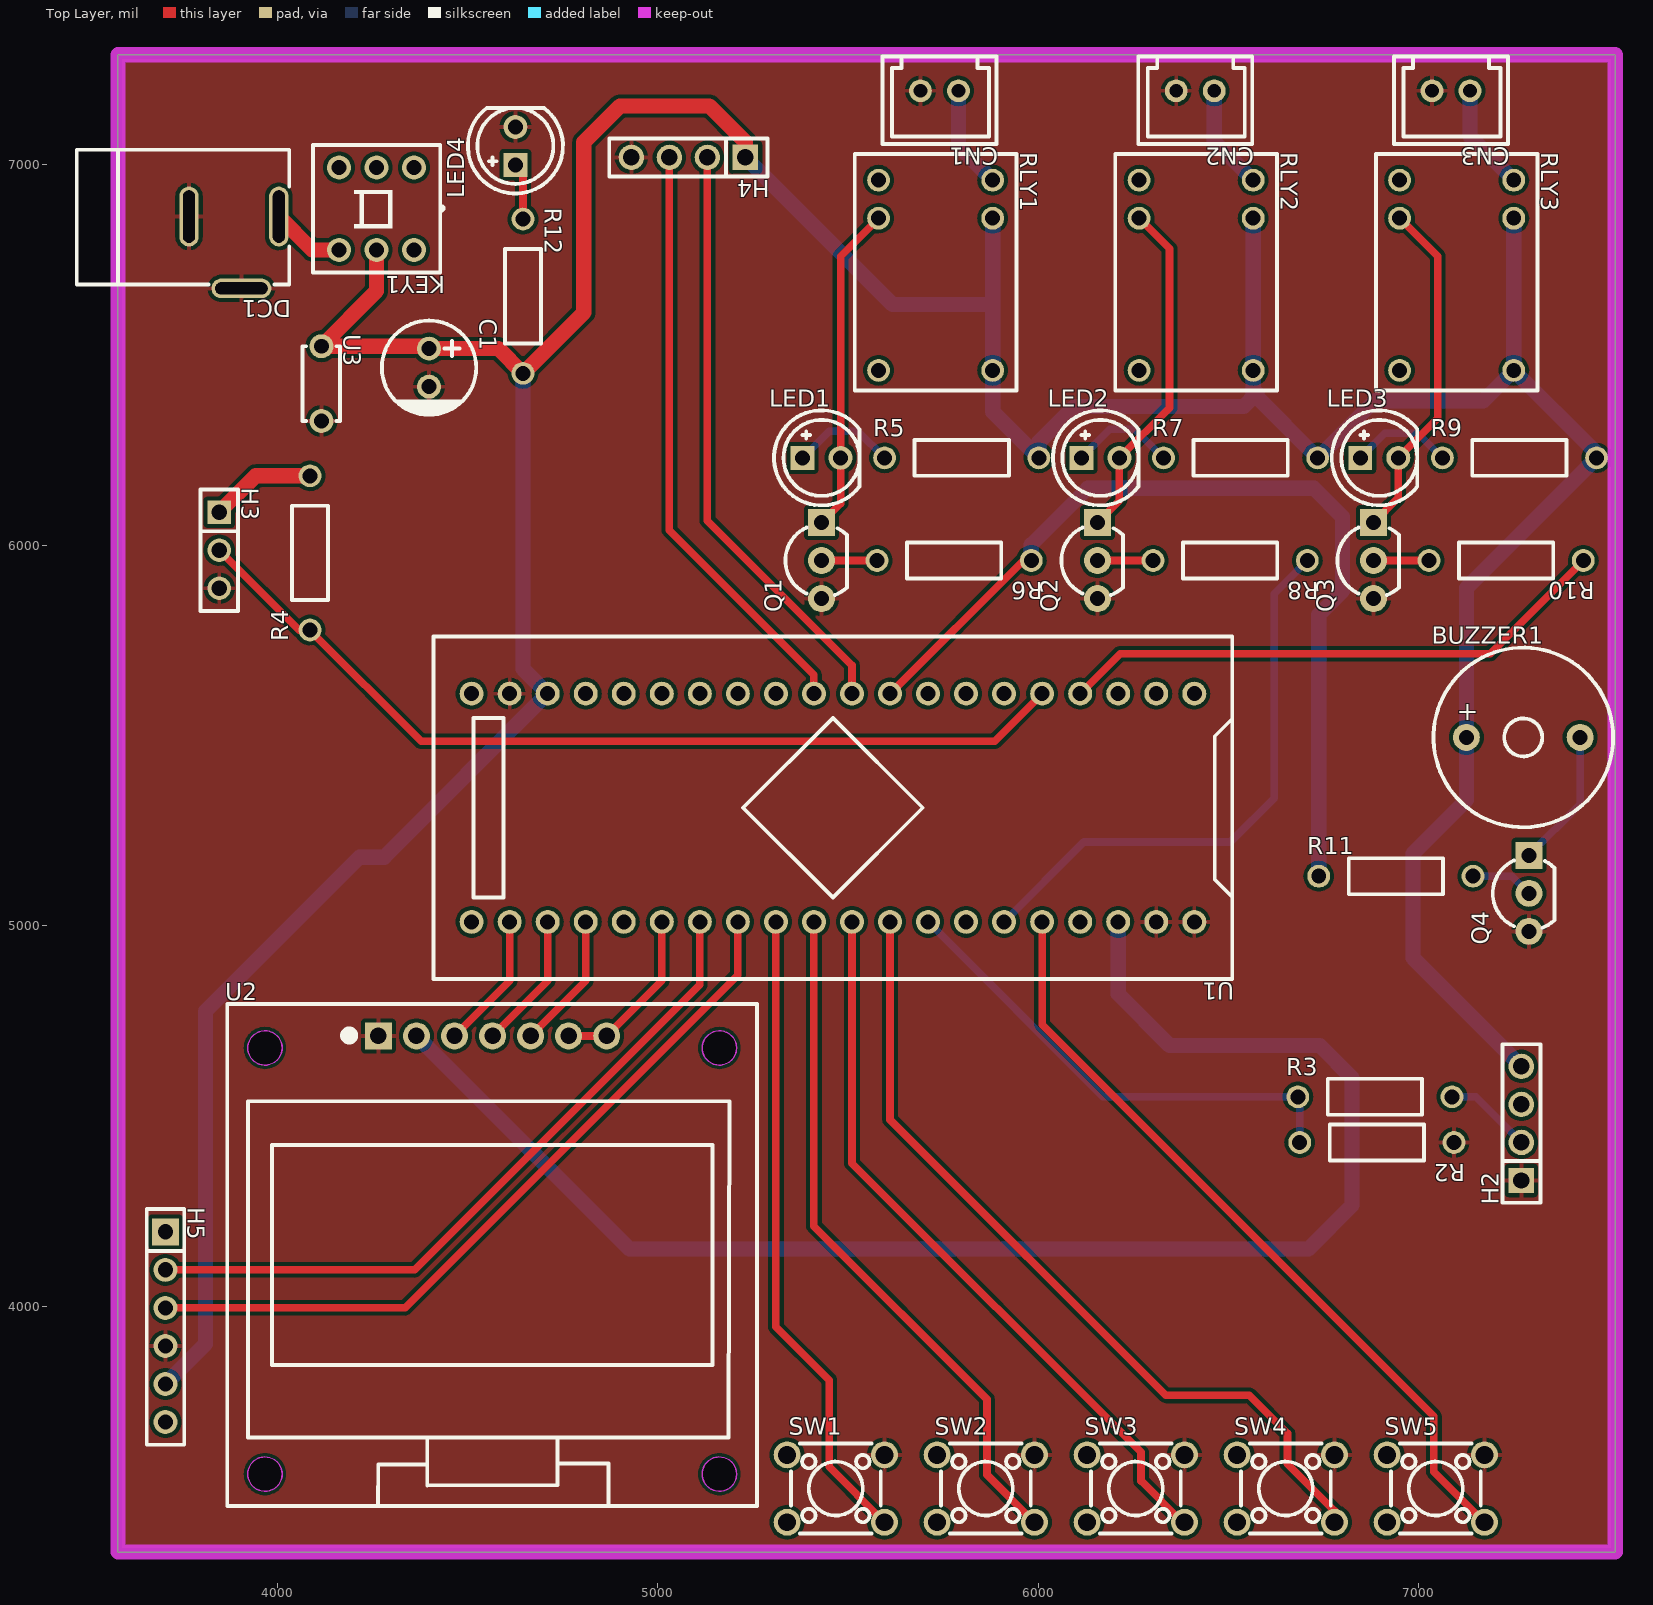
[diagram p0: Top Layer view]
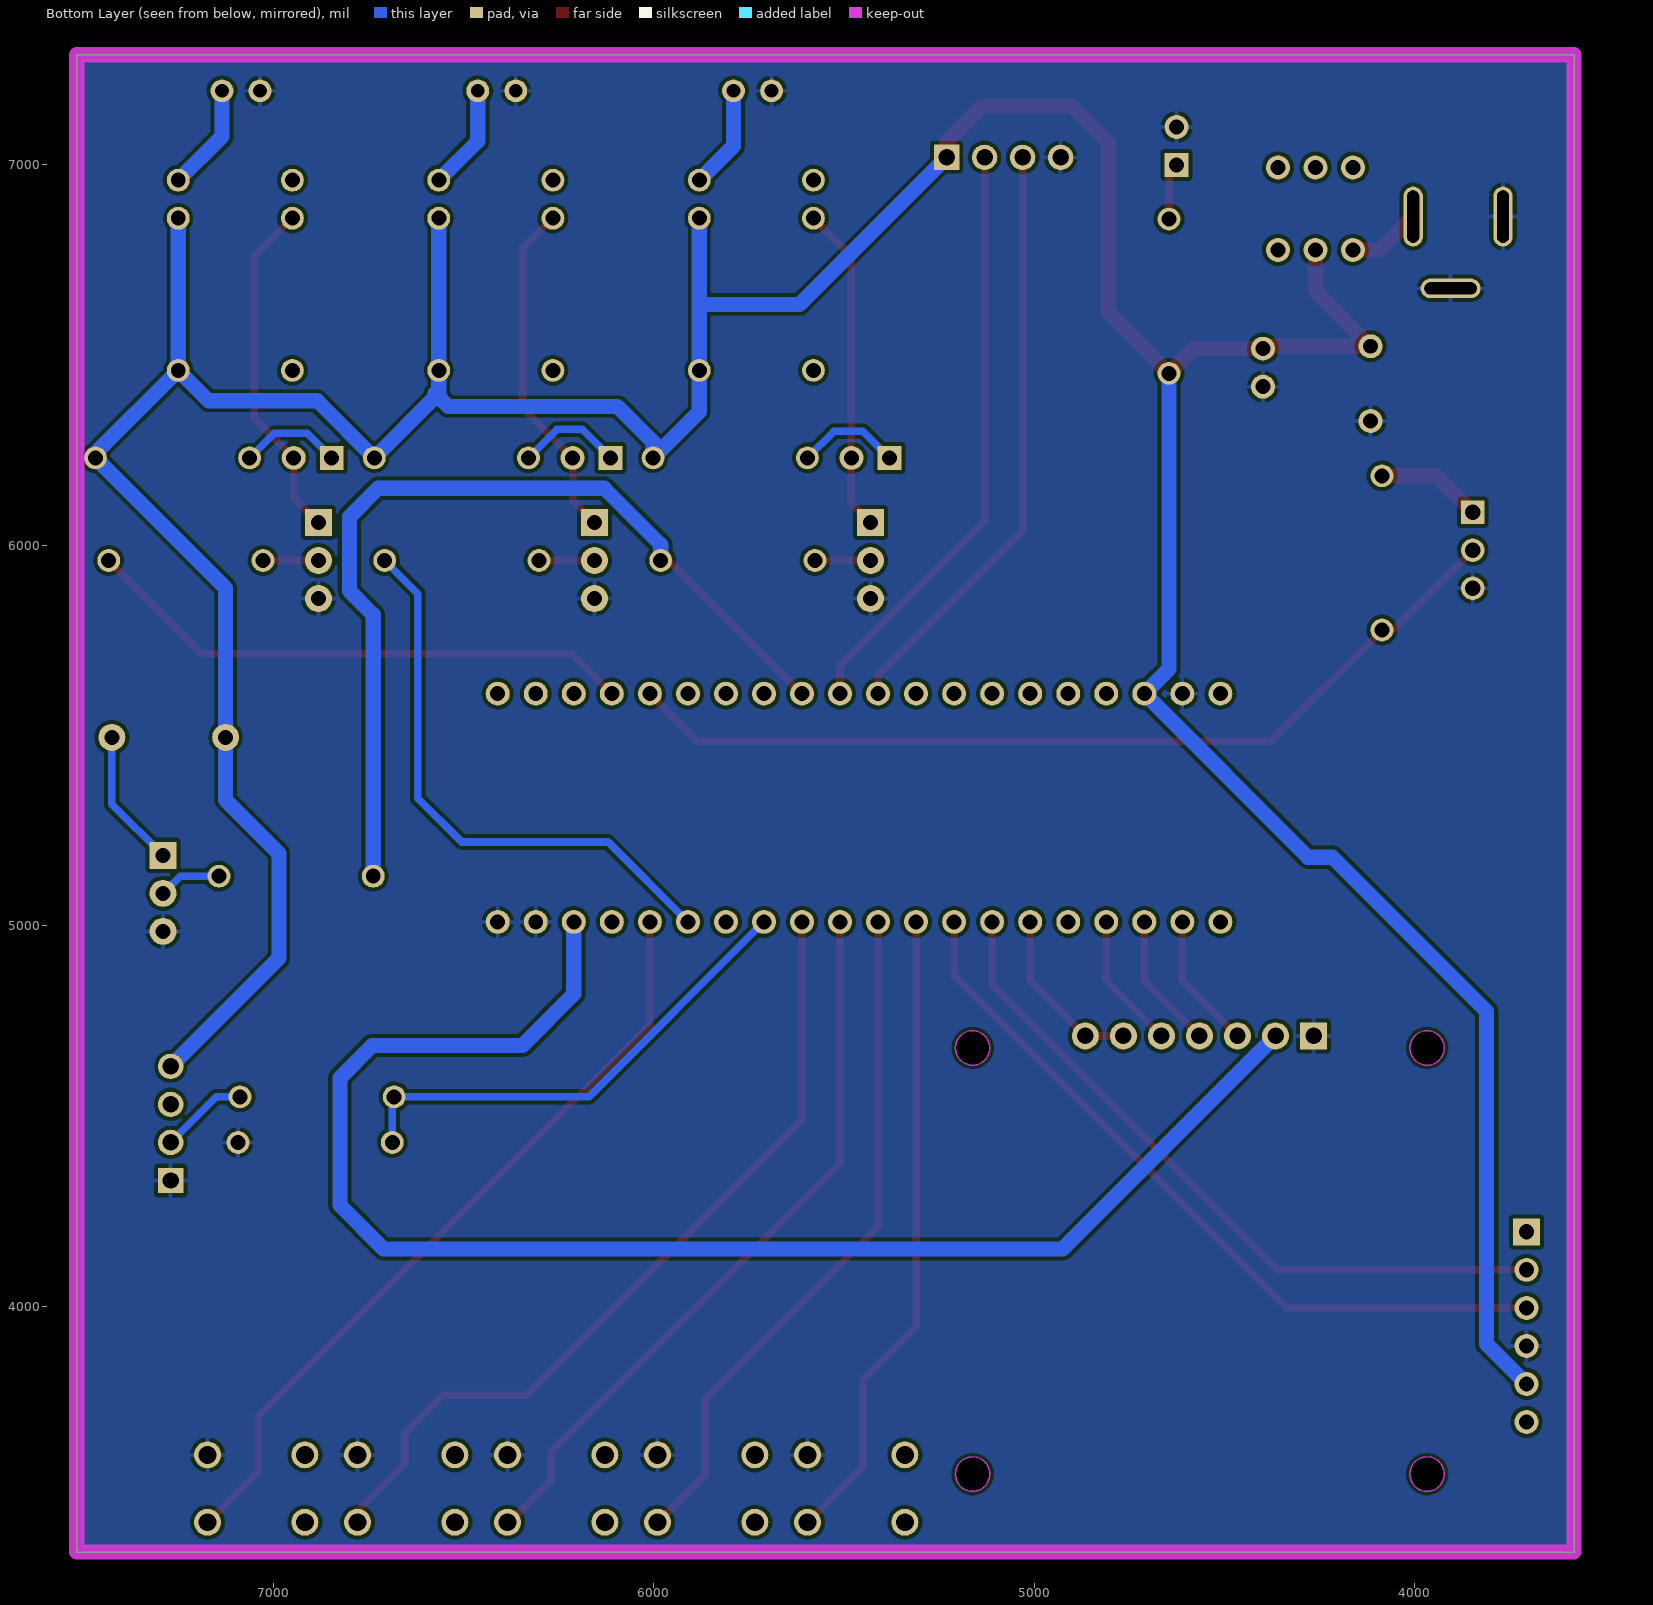
[diagram p1: Bottom Layer view, seen from below]
# Altium PCB MISC50991.pcbdoc
Units mil, origin at the board's own origin, x right, y up, seen from the top; angles counter-clockwise.
Board outline 3937.01 x 3937.01 mil, 2 copper layers (Top Layer, Bottom Layer), stack 62.206 mil thick; 41 components, 56 nets, 165 pads, 0 vias.

## Layer stack, top to bottom
Top Solder Mask Layer: solder mask 0.394, Dk 3.3
Top Layer: signal copper 1.379
Dielectric1: surface 59.449, FR4, Dk 4.5
Bottom Layer: signal copper 1.378
Bottom Solder Mask Layer: solder mask 0.394, Dk 3.3

## Board outline
3580,7290 3580,3352.99 7517.01,3352.99 7517.01,7290

## Design rules (kind name [scope] priority, off if disabled: settings)
BoardOutlineClearance copperThickness2oz_1 [All] p2 off: genericclearance=7.99 ignorepadtopadclearanceinfootprint=FALSE except(0: Arc-SplitContinuation Track-SplitContinuation SMDPad-SplitContinuation THPad-SplitContinuation Via-SplitContinuation Fill-SplitContinuation Region-SplitContinuation Poly-SplitContinuation Text-SplitContinuation Hole-SplitContinuation; 5.98: Arc-CutoutEdge Track-CutoutEdge SMDPad-CutoutEdge THPad-CutoutEdge Via-CutoutEdge Text-CutoutEdge; 6.9: Hole-OutlineEdge Hole-CutoutEdge; 10: Poly-OutlineEdge Poly-CutoutEdge; 11.81: Arc-OutlineEdge Track-OutlineEdge SMDPad-OutlineEdge THPad-OutlineEdge Via-OutlineEdge Fill-OutlineEdge Region-OutlineEdge Text-OutlineEdge Fill-CutoutEdge Region-CutoutEdge)
BoardOutlineClearance Plane_innerPlane_1 [All] p4 off: genericclearance=4.02 ignorepadtopadclearanceinfootprint=FALSE except(0: Arc-SplitContinuation Track-SplitContinuation SMDPad-SplitContinuation THPad-SplitContinuation Via-SplitContinuation Fill-SplitContinuation Region-SplitContinuation Poly-SplitContinuation Text-SplitContinuation Hole-SplitContinuation; 5.98: Arc-CutoutEdge Track-CutoutEdge SMDPad-CutoutEdge THPad-CutoutEdge Via-CutoutEdge Text-CutoutEdge; 6.9: Hole-OutlineEdge Hole-CutoutEdge; 10: Poly-OutlineEdge Poly-CutoutEdge; 11.81: Arc-OutlineEdge Track-OutlineEdge SMDPad-OutlineEdge THPad-OutlineEdge Via-OutlineEdge Fill-OutlineEdge Region-OutlineEdge Text-OutlineEdge Fill-CutoutEdge Region-CutoutEdge)
BoardOutlineClearance Copper_copperRegion_1 [All] p6 off: genericclearance=4.02 ignorepadtopadclearanceinfootprint=FALSE except(0: Arc-SplitContinuation Track-SplitContinuation SMDPad-SplitContinuation THPad-SplitContinuation Via-SplitContinuation Fill-SplitContinuation Region-SplitContinuation Poly-SplitContinuation Text-SplitContinuation Hole-SplitContinuation; 5.98: Arc-CutoutEdge Track-CutoutEdge SMDPad-CutoutEdge THPad-CutoutEdge Via-CutoutEdge Text-CutoutEdge; 6.9: Hole-OutlineEdge Hole-CutoutEdge; 10: Poly-OutlineEdge Poly-CutoutEdge; 11.81: Arc-OutlineEdge Track-OutlineEdge SMDPad-OutlineEdge THPad-OutlineEdge Via-OutlineEdge Fill-OutlineEdge Region-OutlineEdge Text-OutlineEdge Fill-CutoutEdge Region-CutoutEdge)
BoardOutlineClearance copperThickness1oz_1 [All] p8: genericclearance=4.02 ignorepadtopadclearanceinfootprint=FALSE except(0: Arc-SplitContinuation Track-SplitContinuation SMDPad-SplitContinuation THPad-SplitContinuation Via-SplitContinuation Fill-SplitContinuation Region-SplitContinuation Poly-SplitContinuation Text-SplitContinuation Hole-SplitContinuation; 5.98: Arc-CutoutEdge Track-CutoutEdge SMDPad-CutoutEdge THPad-CutoutEdge Via-CutoutEdge Text-CutoutEdge; 6.9: Hole-OutlineEdge Hole-CutoutEdge; 10: Poly-OutlineEdge Poly-CutoutEdge; 11.81: Arc-OutlineEdge Track-OutlineEdge SMDPad-OutlineEdge THPad-OutlineEdge Via-OutlineEdge Fill-OutlineEdge Region-OutlineEdge Text-OutlineEdge Fill-CutoutEdge Region-CutoutEdge)
Clearance copperThickness2oz [All] p1 off: gap=7.99 ignorepadtopadclearanceinfootprint=FALSE except(5.98: SMDPad-Track SMDPad-SMDPad THPad-Track SMDPad-THPad THPad-THPad Track-Via SMDPad-Via THPad-Via Via-Via Fill-SMDPad Region-SMDPad Fill-THPad Region-THPad Fill-Via Region-Via Fill-Fill Fill-Region Region-Region Arc-Track Arc-SMDPad Arc-THPad Arc-Via Fill-Arc Region-Arc Arc-Arc Text-Track SMDPad-Text Text-THPad Text-Via Fill-Text Region-Text Arc-Text Text-Text; 6.9: Hole-Track Hole-SMDPad Hole-THPad Hole-Via Fill-Hole Region-Hole Hole-Arc Hole-Text; 10: Poly-Track Poly-SMDPad Poly-THPad Poly-Via Poly-Fill Poly-Region Poly-Poly Poly-Arc Poly-Text Poly-Hole; 11.81: Fill-Track Region-Track)
Clearance Plane_innerPlane [All] p3 off: gap=4.02 ignorepadtopadclearanceinfootprint=FALSE except(5.98: SMDPad-Track SMDPad-SMDPad THPad-Track SMDPad-THPad THPad-THPad Track-Via SMDPad-Via THPad-Via Via-Via Fill-SMDPad Region-SMDPad Fill-THPad Region-THPad Fill-Via Region-Via Fill-Fill Fill-Region Region-Region Arc-Track Arc-SMDPad Arc-THPad Arc-Via Fill-Arc Region-Arc Arc-Arc Text-Track SMDPad-Text Text-THPad Text-Via Fill-Text Region-Text Arc-Text Text-Text; 6.9: Hole-Track Hole-SMDPad Hole-THPad Hole-Via Fill-Hole Region-Hole Hole-Arc Hole-Text; 10: Poly-Track Poly-SMDPad Poly-THPad Poly-Via Poly-Fill Poly-Region Poly-Poly Poly-Arc Poly-Text Poly-Hole; 11.81: Fill-Track Region-Track)
Clearance Copper_copperRegion [All] p5 off: gap=4.02 ignorepadtopadclearanceinfootprint=FALSE except(5.98: SMDPad-Track SMDPad-SMDPad THPad-Track SMDPad-THPad THPad-THPad Track-Via SMDPad-Via THPad-Via Via-Via Fill-SMDPad Region-SMDPad Fill-THPad Region-THPad Fill-Via Region-Via Fill-Fill Fill-Region Region-Region Arc-Track Arc-SMDPad Arc-THPad Arc-Via Fill-Arc Region-Arc Arc-Arc Text-Track SMDPad-Text Text-THPad Text-Via Fill-Text Region-Text Arc-Text Text-Text; 6.9: Hole-Track Hole-SMDPad Hole-THPad Hole-Via Fill-Hole Region-Hole Hole-Arc Hole-Text; 10: Poly-Track Poly-SMDPad Poly-THPad Poly-Via Poly-Fill Poly-Region Poly-Poly Poly-Arc Poly-Text Poly-Hole; 11.81: Fill-Track Region-Track)
Clearance copperThickness1oz [All] p7: gap=4.02 ignorepadtopadclearanceinfootprint=FALSE except(5.98: SMDPad-Track SMDPad-SMDPad THPad-Track SMDPad-THPad THPad-THPad Track-Via SMDPad-Via THPad-Via Via-Via Fill-SMDPad Region-SMDPad Fill-THPad Region-THPad Fill-Via Region-Via Fill-Fill Fill-Region Region-Region Arc-Track Arc-SMDPad Arc-THPad Arc-Via Fill-Arc Region-Arc Arc-Arc Text-Track SMDPad-Text Text-THPad Text-Via Fill-Text Region-Text Arc-Text Text-Text; 6.9: Hole-Track Hole-SMDPad Hole-THPad Hole-Via Fill-Hole Region-Hole Hole-Arc Hole-Text; 10: Poly-Track Poly-SMDPad Poly-THPad Poly-Via Poly-Fill Poly-Region Poly-Poly Poly-Arc Poly-Text Poly-Hole; 11.81: Fill-Track Region-Track)
DiffPairsRouting differentialPair [All] p1: maxlimit=6 minlimit=6 mostfreqgap=6 toplayer_minwidth=5 toplayer_prefwidth=10 toplayer_maxwidth=100 toplayer_mingap=6 toplayer_prefgap=6 toplayer_maxgap=6 bottomlayer_minwidth=5 bottomlayer_prefwidth=10 bottomlayer_maxwidth=100 bottomlayer_mingap=6 bottomlayer_prefgap=6 bottomlayer_maxgap=6 maxuncoupledlength=10
HoleToHoleClearance otherClearance [All] p1: gap=11.81 allowstackedmicrovias=TRUE
Length netLength [All] p1: minlimit=0 maxlimit=0
PasteMaskExpansion pasteMaskExpansion [All] p1: expansion=0
PlaneConnect innerPlane [All] p1: planeconnectstyle=Relief reliefexpansion=20 reliefentries=4 reliefconductorwidth=10 reliefairgap=10
PolygonConnect copperRegion [All] p1: connectstyle=Relief reliefconductorwidth=10 reliefentries=4 polygonreliefangle="90 Angle" airgapwidth=10 via.connectstyle=Relief via.reliefconductorwidth=10 via.reliefentries=4 via.polygonreliefangle="90 Angle" via.airgapwidth=10
RoutingVias viaSize [All] p1: holewidth=12.01 width=24.02 viastyle="Through Hole" minholewidth=11.81 minwidth=19.68 maxholewidth=248.03 maxwidth=393.7
SolderMaskExpansion solderMaskExpansion [IsVia] p1: expansion=-1000 istentingtop=TRUE
SolderMaskExpansion solderMaskExpansion [All] p2: expansion=2 istentingtop=FALSE
Width copperThickness2oz_2 [All] p1 off: maxlimit=100 minlimit=8 preferedwidth=10
Width copperThickness1oz_2 [All] p2: maxlimit=100 minlimit=5 preferedwidth=10

## Components (designator, comment, footprint, x,y, rotation, side; value= is the part's Value field where it differs from the comment)
BUZZER1 "buzzer-12X9" BUZ-TH_BD12.0-P7.60-D0.6-FD 7275,5495 r0 top
C1 "220uF" CAP-TH_BD6.3-P2.50-D1.0-FD 4398,6467.12 r270 top
CN1 "2P PH2.54" CONN-TH_2P-P2.54_HDR2 5740,7195 r180 top
CN2 "2P PH2.54" CONN-TH_2P-P2.54_HDR2 6412.5,7195 r180 top
CN3 "2P PH2.54" CONN-TH_2P-P2.54_HDR2 7085,7195 r180 top
DC1 "" DC-2.0 3880,6875 r180 top
H2 "" HDR-TH_4P-P2.54-V-F 7270,4480 r90 top
H3 "" HDR-TH_3P-P2.54-V-F 3846.54,5987.12 r270 top
H4 "" HDR-TH_4P-P2.54-V-F 5080,7020 r180 top
H5 "" HDR-TH_6P-P2.54-V-F 3705,3945 r270 top
KEY1 "Non-latching switch 8.5×8.5 silent" SW-TH_6P-L8.5-W8.5-P2.54 4260,6885 r180 top
LED1 "" LED-TH_5mm 5430,6230 r0 top
LED2 "" LED-TH_5mm 6163.21,6230 r0 top
LED3 "" LED-TH_5mm 6896.43,6230 r0 top
LED4 "" LED-TH_5mm 4625,7050 r90 top
Q1 "9013" TO-92-3_L4.8-W3.7-P2.54-R 5430,5960 r90 top
Q2 "9013" TO-92-3_L4.8-W3.7-P2.54-R 6155.64,5960 r90 top
Q3 "9013" TO-92-3_L4.8-W3.7-P2.54-R 6881.29,5960 r90 top
Q4 "9013" TO-92-3_L4.8-W3.7-P2.54-R 7290,5085 r90 top
R2 "10kΩ" Res_1/4W 6890,4430 r180 top
R3 "5kΩ" Res_1/4W 6885,4550 r0 top
R4 "5kΩ" Res_1/4W 4085,5980 r90 top
R5 "5kΩ" Res_1/4W 5798.57,6230 r0 top
R6 "5kΩ" Res_1/4W 5778.71,5960 r180 top
R7 "5kΩ" Res_1/4W 6531.79,6230 r0 top
R8 "5kΩ" Res_1/4W 6504.36,5960 r180 top
R9 "5kΩ" Res_1/4W 7265,6230 r0 top
R10 "5kΩ" Res_1/4W 7230,5960 r180 top
R11 "5kΩ" Res_1/4W 6940,5130 r0 top
R12 "5kΩ" Res_1/4W 4645,6655 r270 top
RLY1 "SRS-05VDC-SL-C" RELAY-TH_SRS-05VDC-SL-C 5730,6710 r270 top
RLY2 "SRS-05VDC-SL-C" RELAY-TH_SRS-05VDC-SL-C 6415,6710 r270 top
RLY3 "SRS-05VDC-SL-C" RELAY-TH_SRS-05VDC-SL-C 7100,6710 r270 top
SW1 "" SW-TH_4P-L6.0-W6.0-P4.50-LS6.5 5467.49,3520 r180 top
SW2 "" SW-TH_4P-L6.0-W6.0-P4.50-LS6.5 5861.87,3520 r180 top
SW3 "" SW-TH_4P-L6.0-W6.0-P4.50-LS6.5 6256.25,3520 r180 top
SW4 "" SW-TH_4P-L6.0-W6.0-P4.50-LS6.5 6650.62,3520 r180 top
SW5 "" SW-TH_4P-L6.0-W6.0-P4.50-LS6.5 7045,3520 r180 top
U1 "STM32F103C8T6-Card" CONN-TH_L53.3-W22.9_STM32F103C8T6-CARD 5460,5310 r180 top
U2 "1.30OLED_7P" LCD-TH_7P-P2.54_1.30OLED_7P 4565,4710 r0 top
U3 "100nF" CAP-TH_L5.0-W2.5-P5.00-D1.0 4115,6425 r270 top

## Footprints (in the part's own frame and the unit in brackets; to place one, negate y for a bottom-side part, rotate by r counter-clockwise, add the part's x,y. Pads: shape width x height; smd on the part's side, far side on the other; paste and mask are expansions set on the pad)
BUZ-TH_BD12.0-P7.60-D0.6-FD [mm]
  round 1.8 hole 1: 1(-3.8,0) 2(3.8,0)
  silkscreen extent -6,-6 6,6
CAP-TH_BD6.3-P2.50-D1.0-FD [mm]
  round 1.6 hole 1: 1(-1.27,0) 2(1.27,0)
  silkscreen extent -3.15,-3.15 3.17,3.15
CAP-TH_L5.0-W2.5-P5.00-D1.0 [mm]
  round 1.6 hole 1: 1(-2.5,0) 2(2.5,0)
  silkscreen extent -2.5,-1.27 2.5,1.25
CONN-TH_2P-P2.54_HDR2 [mil]
  round 60 hole 36 paste+0 mask+1.97: 1(-50,0) 2(50,0)
  silkscreen extent -150,-90 150,140
CONN-TH_L53.3-W22.9_STM32F103C8T6-CARD [mm]
  round 1.6 hole 1: 1(-24.13,-7.62) 2(-21.59,-7.62) 3(-19.05,-7.62) 4(-16.51,-7.62) 5(-13.97,-7.62) 6(-11.43,-7.62) 7(-8.89,-7.62) 8(-6.35,-7.62) 9(-3.81,-7.62) 10(-1.27,-7.62) 11(1.27,-7.62) 12(3.81,-7.62) 13(6.35,-7.62) 14(8.89,-7.62) 15(11.43,-7.62) 16(13.97,-7.62) 17(16.51,-7.62) 18(19.05,-7.62) 19(21.59,-7.62) 20(24.13,-7.62) 21(24.13,7.62) 22(21.59,7.62) 23(19.05,7.62) 24(16.51,7.62) 25(13.97,7.62) 26(11.43,7.62) 27(8.89,7.62) 28(6.35,7.62) 29(3.81,7.62) 30(1.27,7.62) 31(-1.27,7.62) 32(-3.81,7.62) 33(-6.35,7.62) 34(-8.89,7.62) 35(-11.43,7.62) 36(-13.97,7.62) 37(-16.51,7.62) 38(-19.05,7.62) 39(-21.59,7.62) 40(-24.13,7.62)
  silkscreen extent -26.67,-11.43 26.67,11.43
DC-2.0 [mil]
  oval 157.5x51.2 hole 31.5 slot 137.8 at 0 deg paste+0 mask+2: 2(-24.7,199.5)
  oval 51.2x157.5 hole 31.5 slot 137.8 at 90 deg paste+0 mask+2: 3(113.1,10.5) 4(-123.1,10.5)
  silkscreen extent -151,-165 408,190
HDR-TH_3P-P2.54-V-F [mil]
  rect 62x62 hole 40.16: 1(-100,0)
  round 62 hole 40.16: 2(0,0) 3(100,0)
  silkscreen extent -160,-49 160,49
HDR-TH_4P-P2.54-V-F [mm]
  rect 1.7x1.7 hole 1.1: 1(-3.81,0)
  round 1.7 hole 1.1: 2(-1.27,0) 3(1.27,0) 4(3.81,0)
  silkscreen extent -5.29,-1.27 5.29,1.27
HDR-TH_6P-P2.54-V-F [mm]
  rect 1.8x1.8 hole 1.02: 1(-6.35,0)
  round 1.6 hole 1.02: 2(-3.81,0) 3(-1.27,0) 4(1.27,0) 5(3.81,0) 6(6.35,0)
  silkscreen extent -7.87,-1.25 7.87,1.25
LCD-TH_7P-P2.54_1.30OLED_7P [mil]
  rect 70.94x70.94 hole 43.3: 1(-300,-0.01)
  round 70.94 hole 43.3: 2(-200,-0.01) 3(-100,-0.01) 4(0,-0.01) 5(100,-0.01) 6(200,-0.01) 7(300,-0.01)
  Board Outline Layer circle w0.1: c-598.44,-31.49 r45.28
  Board Outline Layer circle w0.1: c596.44,-1151.96 r45.28
  Board Outline Layer circle w0.1: c596.44,-31.49 r45.28
  Board Outline Layer circle w0.1: c-598.44,-1151.96 r45.28
  Board Outline Layer region: -553.17,-31.49 -557.65,-51.14 -570.21,-66.89 -588.37,-75.63 -608.52,-75.63 -626.67,-66.89 -639.23,-51.14 -643.72,-31.49 -643.72,-31.49 -639.23,-11.85 -626.67,3.91 -608.52,12.65 -588.37,12.65 -570.21,3.91 -557.65,-11.85 -553.17,-31.49
  Board Outline Layer region: -553.17,-31.49 -553.55,-37.4 -554.71,-43.21 -556.61,-48.82 -559.23,-54.13 -562.52,-59.06 -566.43,-63.51 -570.88,-67.41 -575.8,-70.7 -581.12,-73.32 -586.72,-75.23 -592.53,-76.38 -598.44,-76.77 -604.35,-76.38 -610.16,-75.23 -615.77,-73.32 -621.08,-70.7 -626,-67.41 -630.46,-63.51 -634.36,-59.06 -637.65,-54.13 -640.27,-48.82 -642.18,-43.21 -643.33,-37.4 -643.72,-31.49 -643.33,-25.58 -642.18,-19.77 -640.27,-14.17 -637.65,-8.85 -634.36,-3.93 -630.46,0.52 -626,4.43 -621.08,7.72 -615.77,10.34 -610.16,12.24 -604.35,13.4 -598.44,13.78 -592.53,13.4 -586.72,12.24 -581.12,10.34 -575.8,7.72 -570.88,4.43 -566.43,0.52 -562.52,-3.93 -559.23,-8.85 -556.61,-14.17 -554.71,-19.77 -553.55,-25.58
  Board Outline Layer region: 641.71,-1151.96 637.23,-1171.61 624.67,-1187.36 606.51,-1196.1 586.36,-1196.1 568.21,-1187.36 555.65,-1171.61 551.16,-1151.96 551.16,-1151.96 555.65,-1132.32 568.21,-1116.56 586.36,-1107.82 606.51,-1107.82 624.67,-1116.56 637.23,-1132.32 641.71,-1151.96
  Board Outline Layer region: 641.71,-1151.96 641.33,-1157.87 640.17,-1163.68 638.27,-1169.29 635.65,-1174.6 632.36,-1179.53 628.45,-1183.98 624,-1187.88 619.08,-1191.17 613.76,-1193.79 608.16,-1195.7 602.35,-1196.85 596.44,-1197.24 590.53,-1196.85 584.72,-1195.7 579.11,-1193.79 573.8,-1191.17 568.88,-1187.88 564.42,-1183.98 560.52,-1179.53 557.23,-1174.6 554.61,-1169.29 552.7,-1163.68 551.55,-1157.87 551.16,-1151.96 551.55,-1146.05 552.7,-1140.24 554.61,-1134.64 557.23,-1129.32 560.52,-1124.4 564.42,-1119.95 568.88,-1116.04 573.8,-1112.75 579.11,-1110.13 584.72,-1108.23 590.53,-1107.07 596.44,-1106.69 602.35,-1107.07 608.16,-1108.23 613.76,-1110.13 619.08,-1112.75 624,-1116.04 628.45,-1119.95 632.36,-1124.4 635.65,-1129.32 638.27,-1134.64 640.17,-1140.24 641.33,-1146.05
  Board Outline Layer region: 641.71,-31.49 637.23,-51.14 624.67,-66.89 606.51,-75.63 586.36,-75.63 568.21,-66.89 555.65,-51.14 551.16,-31.49 551.16,-31.49 555.65,-11.85 568.21,3.91 586.36,12.65 606.51,12.65 624.67,3.91 637.23,-11.85 641.71,-31.49
  Board Outline Layer region: 641.71,-31.49 641.33,-37.4 640.17,-43.21 638.27,-48.82 635.65,-54.13 632.36,-59.06 628.45,-63.51 624,-67.41 619.08,-70.7 613.76,-73.32 608.16,-75.23 602.35,-76.38 596.44,-76.77 590.53,-76.38 584.72,-75.23 579.11,-73.32 573.8,-70.7 568.88,-67.41 564.42,-63.51 560.52,-59.06 557.23,-54.13 554.61,-48.82 552.7,-43.21 551.55,-37.4 551.16,-31.49 551.55,-25.58 552.7,-19.77 554.61,-14.17 557.23,-8.85 560.52,-3.93 564.42,0.52 568.88,4.43 573.8,7.72 579.11,10.34 584.72,12.24 590.53,13.4 596.44,13.78 602.35,13.4 608.16,12.24 613.76,10.34 619.08,7.72 624,4.43 628.45,0.52 632.36,-3.93 635.65,-8.85 638.27,-14.17 640.17,-19.77 641.33,-25.58
  Board Outline Layer region: -553.17,-1151.96 -557.65,-1171.61 -570.21,-1187.36 -588.37,-1196.1 -608.52,-1196.1 -626.67,-1187.36 -639.23,-1171.61 -643.72,-1151.96 -643.72,-1151.96 -639.23,-1132.32 -626.67,-1116.56 -608.52,-1107.82 -588.37,-1107.82 -570.21,-1116.56 -557.65,-1132.32 -553.17,-1151.96
  Board Outline Layer region: -553.17,-1151.96 -553.55,-1157.87 -554.71,-1163.68 -556.61,-1169.29 -559.23,-1174.6 -562.52,-1179.53 -566.43,-1183.98 -570.88,-1187.88 -575.8,-1191.17 -581.12,-1193.79 -586.72,-1195.7 -592.53,-1196.85 -598.44,-1197.24 -604.35,-1196.85 -610.16,-1195.7 -615.77,-1193.79 -621.08,-1191.17 -626,-1187.88 -630.46,-1183.98 -634.36,-1179.53 -637.65,-1174.6 -640.27,-1169.29 -642.18,-1163.68 -643.33,-1157.87 -643.72,-1151.96 -643.33,-1146.05 -642.18,-1140.24 -640.27,-1134.64 -637.65,-1129.32 -634.36,-1124.4 -630.46,-1119.95 -626,-1116.04 -621.08,-1112.75 -615.77,-1110.13 -610.16,-1108.23 -604.35,-1107.07 -598.44,-1106.69 -592.53,-1107.07 -586.72,-1108.23 -581.12,-1110.13 -575.8,-1112.75 -570.88,-1116.04 -566.43,-1119.95 -562.52,-1124.4 -559.23,-1129.32 -556.61,-1134.64 -554.71,-1140.24 -553.55,-1146.05
  Multi-Layer board cut-out: -553.17,-31.49 -557.65,-51.14 -570.21,-66.89 -588.37,-75.63 -608.52,-75.63 -626.67,-66.89 -639.23,-51.14 -643.72,-31.49 -643.72,-31.49 -639.23,-11.85 -626.67,3.91 -608.52,12.65 -588.37,12.65 -570.21,3.91 -557.65,-11.85 -553.17,-31.49
  Multi-Layer board cut-out: 641.71,-1151.96 637.23,-1171.61 624.67,-1187.36 606.51,-1196.1 586.36,-1196.1 568.21,-1187.36 555.65,-1171.61 551.16,-1151.96 551.16,-1151.96 555.65,-1132.32 568.21,-1116.56 586.36,-1107.82 606.51,-1107.82 624.67,-1116.56 637.23,-1132.32 641.71,-1151.96
  Multi-Layer board cut-out: 641.71,-31.49 637.23,-51.14 624.67,-66.89 606.51,-75.63 586.36,-75.63 568.21,-66.89 555.65,-51.14 551.16,-31.49 551.16,-31.49 555.65,-11.85 568.21,3.91 586.36,12.65 606.51,12.65 624.67,3.91 637.23,-11.85 641.71,-31.49
  Multi-Layer board cut-out: -553.17,-1151.96 -557.65,-1171.61 -570.21,-1187.36 -588.37,-1196.1 -608.52,-1196.1 -626.67,-1187.36 -639.23,-1171.61 -643.72,-1151.96 -643.72,-1151.96 -639.23,-1132.32 -626.67,-1116.56 -608.52,-1107.82 -588.37,-1107.82 -570.21,-1116.56 -557.65,-1132.32 -553.17,-1151.96
  silkscreen extent -697,-1236 695,84
LED-TH_5mm [mm]
  rect 1.6x1.6 hole 1 paste+0 mask+0.051: 1(-1.27,0)
  round 1.6 hole 1 paste+0 mask+0.051: 2(1.27,0)
  silkscreen extent -3.17,-3.17 2.54,3.17
RELAY-TH_SRS-05VDC-SL-C [mil]
  round 60 hole 39.37: 1(-250,150) 2(-150,150) 3(250,150) 4(250,-150) 5(-150,-150) 6(-250,-150)
  silkscreen extent -319,-213 303,213
Res_1/4W [mil]
  round 60 hole 39.37 paste+0 mask+2: 1(-202.76,0) 2(202.76,0)
  silkscreen extent -124,-47 124,47
SW-TH_4P-L6.0-W6.0-P4.50-LS6.5 [mm]
  round 1.8 hole 1.2: 1(-3.25,2.25) 2(3.25,2.25) 3(-3.25,-2.25) 4(3.25,-2.25)
  silkscreen extent -3,-3 3,3
SW-TH_6P-L8.5-W8.5-P2.54 [mm]
  round 1.6 hole 1: 1(-2.5,-2.75) 2(0,-2.75) 3(2.5,-2.75) 4(-2.5,2.75) 5(0,2.75) 6(2.5,2.75)
  silkscreen extent -4.47,-4.25 4.25,4.25
TO-92-3_L4.8-W3.7-P2.54-R [mm]
  rect 1.8x1.8 hole 1: 1(2.54,0)
  round 1.8 hole 1: 2(0,0) 3(-2.54,0)
  silkscreen extent -2.3,-1.7 2.2,2.41

## Nets (pads, with @x,y where several pads share a name; then routed paths per layer and width w, separated by ;. In a path a pad name is that pad's centre, name@x,y a point inside that pad or via, vN(x,y) a via of type N, cw(c..) or ccw(c..) an arc to the next point about the centre after c; other vN are vias at no path point)
3V3: U1.38 U2.2 | length 3970.7
  Bottom Layer w40: U2.2 4924.99,4150 6710,4150 6825,4265 6825,4600 6740,4685 6345,4685 6210,4820 U1.38
$1N851: H2.2 R3.2 | length 231.9
  Bottom Layer w20: R3.2 7150,4550 H2.2
$1N1036: H3.1 R4.2 | length 278.1
  Top Layer w40: H3.1 3942.18,6182.76 R4.2
$1N1532: LED1.1 R5.1 | length 273.8
  Bottom Layer w20: LED1.1 5450,6300 5525.81,6300 R5.1
$1N1605: LED1.2 Q1.1 RLY1.5 | length 862.1
  Top Layer w20: Q1.1 5480,6110 LED1.2 5480,6760 RLY1.5
$1N1711: Q1.2 R6.2 | length 146
  Top Layer w20: Q1.2 R6.2
$1N1775: CN1.1 RLY1.1 | length 272.3
  Bottom Layer w40: CN1.1 5790,7050 RLY1.1
$1N2029: LED2.1 R7.1 | length 277.9
  Bottom Layer w20: LED2.1 6188.21,6305 6254.03,6305 R7.1
$1N2031: LED2.2 Q2.1 RLY2.5 | length 911.6
  Top Layer w20: Q2.1 6213.21,6117.57 LED2.2 6345,6361.79 6345,6780 RLY2.5
$1N2035: Q2.2 R8.2 | length 146
  Top Layer w20: Q2.2 R8.2
$1N2037: CN2.1 RLY2.1 | length 277.5
  Bottom Layer w40: CN2.1 6462.5,7062.5 RLY2.1
$1N2257: LED3.1 R9.1 | length 269.7
  Bottom Layer w20: LED3.1 6911.43,6295 6997.24,6295 R9.1
$1N2259: LED3.2 Q3.1 RLY3.5 | length 911.3
  Top Layer w20: Q3.1 6946.43,6125.14 LED3.2 7050,6333.57 7050,6760 RLY3.5
$1N2263: Q3.2 R10.2 | length 146
  Top Layer w20: Q3.2 R10.2
$1N2265: CN3.1 RLY3.1 | length 282.6
  Bottom Layer w40: CN3.1 7135,7075 RLY3.1
$1N2357: Q4.2 R11.2 | length 165.9
  Bottom Layer w20: R11.2 7245,5130 Q4.2
$1N2427: BUZZER1.2 Q4.1 | length 365.8
  Bottom Layer w20: Q4.1 7424.6,5319.6 BUZZER1.2
$1N3694: DC1.4 KEY1.6 | length 194.8
  Top Layer w40: DC1.4 4090.87,6776.73 KEY1.6
$1N3785: LED4.1 R12.1 | length 150.5
  Top Layer w20: LED4.1 4645,6980 R12.1
+5V: BUZZER1.1 C1.1 H2.4 H4.1 H5.5 KEY1.5 R5.2 R7.2 R9.2 R12.2 RLY1.2 RLY1.3 RLY2.2 RLY2.3 RLY3.2 RLY3.3 U1.18 U3.1 | length 11336.9
  Top Layer w40: KEY1.5 4260.01,6668.43 U3.1 4391.7,6523.43 C1.1 4580.12,6517.12 R12.2 4805,6612.24 4805,7060 4900,7155 5135,7155 5230,7060 H4.1
  Bottom Layer w40: H5.5 3810,3900 3810,4775 4215,5180 4280,5180 U1.18 4645,5675 R12.2 ; H4.1 5616.55,6633.45 5880,6633.45 ; RLY1.2 5880,6633.45 ; RLY2.2 RLY2.3 6565,6399.55 6569.77,6394.77 ; 6575,6400 6569.77,6394.77 ; RLY3.2 RLY3.3 ; H2.4 6985,4915 6985,5190 7125.4,5330.4 BUZZER1.1 7125.4,5887.64 R9.2 7467.76,6242.24 RLY3.3 ; 5880,6633.45 RLY1.3 5880,6351.33 R5.2 6001.33,6271.33 6095,6365 6540,6365 6569.77,6394.77 ; 6569.77,6394.77 R7.2 6884.55,6380 7170,6380 RLY3.3
GND: C1.2 CN1.2 CN2.2 CN3.2 DC1.2 DC1.3 H2.1 H3.3 H4.4 H5.4 LED4.2 Q1.3 Q2.3 Q3.3 Q4.3 R2.1 SW1.3 SW2.3 SW3.3 SW4.3 SW5.3 U1.19 U1.39 U1.40 U2.1 U3.2
NRST: U1.37
PA0: U1.25
PA1: U1.26 U2.6 U2.7 | length 460.1
  Top Layer w20: U2.6 U2.7 5010,4855 U1.26
PA2: H5.2 U1.27 | length 1880.7
  Top Layer w20: H5.2 4360,4095 5110,4845 U1.27
PA3: H5.3 U1.28 | length 2007.4
  Top Layer w20: H5.3 4335,3995 5210,4870 U1.28
PA4: SW1.1 U1.29 | length 1696.8
  Top Layer w20: U1.29 5310,3945 5450,3805 5450,3576.86 SW1.1
PA5: SW2.1 U1.30 | length 1818.7
  Top Layer w20: U1.30 5410,4210 5865,3755 5865,3556.24 SW2.1
PA6: SW3.1 U1.31 | length 1944
  Top Layer w20: U1.31 5510,4375 6270,3615 6270,3540 6378.58,3431.42 SW3.1
PA7: SW4.1 U1.32 | length 2191.5
  Top Layer w20: U1.32 5610,4490 6335,3765 6555,3765 6655,3665 6655,3585 6778.57,3461.43 SW4.1
PA8: H3.2 R4.1 U1.5 | length 2423.2
  Top Layer w20: H3.2 4056.42,5777.24 R4.1 4377.24,5485 5885,5485 U1.5
PA9: U1.6
PA10: U1.7
PA11: U1.8
PA12: R6.1 R11.1 U1.9 | length 2440
  Top Layer w20: U1.9 5960,5960 R6.1
  Bottom Layer w40: R6.1 5981.47,6001.47 6130,6150 6725,6150 6800,6075 6800,5880 6737.24,5817.24 R11.1
PA15: H4.2 U1.10 | length 1567.4
  Top Layer w20: H4.2 5130,6065 5510,5685 U1.10
PB0: R2.2 R3.1 U1.33 | length 1284.9
  Bottom Layer w20: U1.33 6170,4550 R3.1 6687.24,4545 R2.2
PB1: U1.34
PB3: H4.3 U1.11 | length 1567.4
  Top Layer w20: H4.3 5030,6040 5410,5660 U1.11
PB4: U1.12
PB5: U1.13
PB6: U1.14
PB7: U1.15
PB8: U1.16
PB9: U1.17
PB10: R8.1 U1.35 | length 1505.7
  Bottom Layer w20: U1.35 6120,5220 6505,5220 6620,5335 6620,5872.88 R8.1
PB11: SW5.1 U1.36 | length 2060.3
  Top Layer w20: U1.36 6010,4740 7040,3710 7040,3564.37 SW5.1
PB12: U1.1
PB13: U1.2
PB14: U1.3
PB15: R10.1 U1.4 | length 1467.7
  Top Layer w20: U1.4 6215,5715 7187.76,5715 R10.1
PC13: U1.22 U2.3 | length 360.1
  Top Layer w20: U2.3 4610,4855 U1.22
PC14: U1.23 U2.4 | length 360.1
  Top Layer w20: U2.4 4710,4855 U1.23
PC15: U1.24 U2.5 | length 360.1
  Top Layer w20: U2.5 4810,4855 U1.24
VBAT: U1.21
VCC3V3: U1.20
pads on no net: H2.3 H5.1 H5.6 KEY1.1 KEY1.2 KEY1.3 KEY1.4 RLY1.4 RLY1.6 RLY2.4 RLY2.6 RLY3.4 RLY3.6 SW1.2 SW1.4 SW2.2 SW2.4 SW3.2 SW3.4 SW4.2 SW4.4 SW5.2 SW5.4

## Polygon pours and split planes (outlines as drawn)
GND on Top Layer (solid, remove dead copper, pour order 0): 3000,7765 3000,3000 7915,3000 7915,7765
GND on Bottom Layer (solid, remove dead copper, pour order 2): 3195,7520 3195,3105 7655,3105 7655,7520

## Keep-outs
Board Outline Layer:
  the board outline again, w40